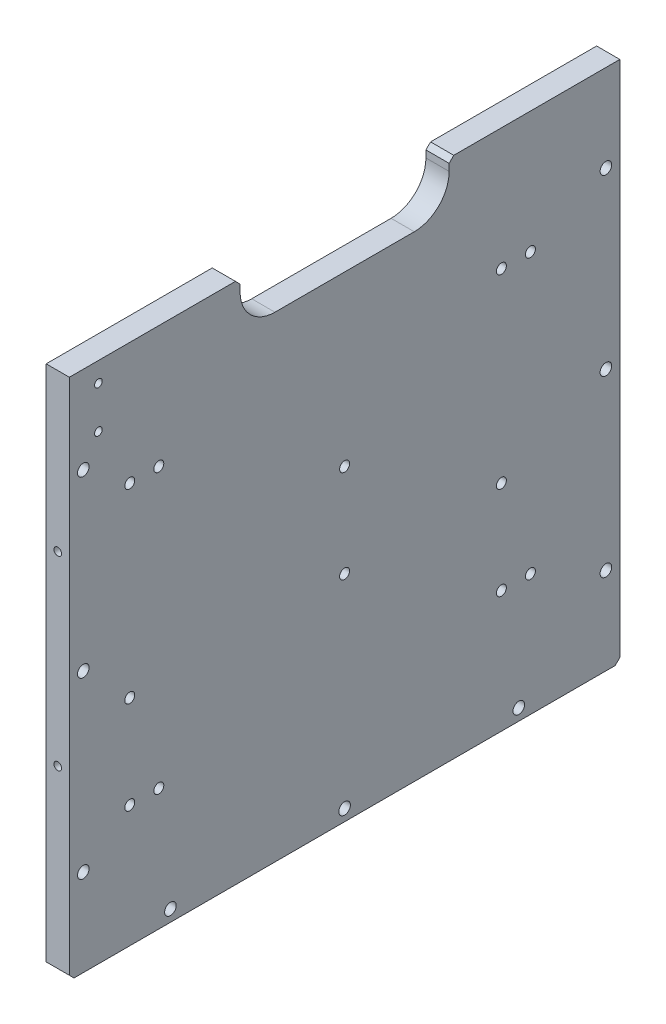
from build123d import *

# Parameters (mm, degrees)
SKETCH_1_W                  = 237
SKETCH_1_H                  = 250
EXTRUDE_1_DEPTH             = 5
MOVE_FACE_1_BY              = 17.5
MOVE_FACE_2_BY              = 7.5
HOLE_WIZARD_M4_1_AT_2_COUNT = 2
HOLE_WIZARD_M4_1_AT_2_PITCH = 80
HOLE_WIZARD_M4_2_D          = 3.3
HOLE_WIZARD_M6_1_D          = 5
HOLE_WIZARD_M6_2_D          = 5
CHAMFER_1_SIZE              = 2
CUT_EXTRUDE_1_DEPTH         = 71
CHAMFER_2_SIZE              = 2
HOLE_WIZARD_1_D             = 4.3
HOLE_WIZARD_1_CBORE_D       = 8
HOLE_WIZARD_1_CBORE_DEPTH   = 4.6
HOLE_WIZARD_1_2_D           = 4.3
HOLE_WIZARD_1_2_CBORE_D     = 8
HOLE_WIZARD_1_2_CBORE_DEPTH = 5


with BuildPart() as part:
    # 草图1 → 凸台-拉伸1 (new, symmetric)
    with BuildSketch(Plane(origin=(0, 0, 0), x_dir=(0, 0, -1), z_dir=(1, 0, 0))):
        Rectangle(SKETCH_1_W, SKETCH_1_H)
    extrude(amount=EXTRUDE_1_DEPTH, both=True)

    # Move Face 1: a face moved inward by 17.5
    extrude(part.faces().sort_by_distance((0, 125, 0))[0], amount=MOVE_FACE_1_BY, dir=(0, -1, 0), mode=Mode.SUBTRACT)

    # Move Face 2: a face moved inward by 7.5
    extrude(part.faces().sort_by_distance((0, -125, 0))[0], amount=MOVE_FACE_2_BY, dir=(0, 1, 0), mode=Mode.SUBTRACT)

    # 草图3 → M4 螺纹孔1 (revolve, cut)
    with BuildSketch(Plane(origin=(0, -40, 118.5), x_dir=(0, -1, 0), z_dir=(1, 0, 0))):
        Polygon((0, 0), (0, 11.091420021), (1.65, 10.1), (1.65, 0), align=None)
    hole_wizard_m4_1 = revolve(axis=Axis((0, -40, 124.85), (0, 0, -1)), mode=Mode.SUBTRACT)

    # M4 螺纹孔1 at 2: M4 螺纹孔1 ×2
    with Locations(*[(0, i * HOLE_WIZARD_M4_1_AT_2_PITCH, 0) for i in range(1, HOLE_WIZARD_M4_1_AT_2_COUNT)]):
        add(hole_wizard_m4_1, mode=Mode.SUBTRACT)

    # 镜向1: M4 螺纹孔1 across plane
    add(hole_wizard_m4_1.mirror(Plane.XY), mode=Mode.SUBTRACT)

    # 镜向1 copy 1 sketch → 镜向1 copy 1 (revolve, cut)
    with BuildSketch(Plane(origin=(0, 40, -118.5), x_dir=(0, -1, 0), z_dir=(1, 0, 0))):
        Polygon((0, 0), (0, -11.091420021), (1.65, -10.1), (1.65, 0), align=None)
    revolve(axis=Axis((0, 40, -124.85), (0, 0, -1)), mode=Mode.SUBTRACT)

    # M4 螺纹孔2 (through all)
    with Locations(Plane(origin=(5, 0, 0), x_dir=(0, 0, -1), z_dir=(1, 0, 0))):
        with Locations((-106, 99), (-106, 81)):
            Hole(HOLE_WIZARD_M4_2_D / 2)

    # M6 螺纹孔1 (through all)
    with Locations(Plane.ZY.offset(5)):
        with Locations((-112.5, 70), (-112.5, -5), (-112.5, -80)):
            hole_wizard_m6_1 = Hole(HOLE_WIZARD_M6_1_D / 2)

    # 镜向2: M6 螺纹孔1 across plane
    add(hole_wizard_m6_1.mirror(Plane.XY), mode=Mode.SUBTRACT)

    # M6 螺纹孔2 (through all)
    with Locations(Plane.ZY.offset(5)):
        with Locations((75, -112.5), (0, -112.5), (-75, -112.5)):
            Hole(HOLE_WIZARD_M6_2_D / 2)

    # 倒角1
    chamfer_1_edges = [part.edges().sort_by_distance(p)[0] for p in [
        (0, -117.5, -118.5),
        (0, -117.5, 118.5),
    ]]
    chamfer(chamfer_1_edges, length=CHAMFER_1_SIZE)

    # 草图11 → 切除-拉伸1 (cut)
    with BuildSketch(Plane.ZY.offset(5)):
        with BuildLine():
            Line((-45, 148.579976686), (45, 148.579976686))
            Line((45, 148.579976686), (45, 102.5))
            ThreePointArc((45, 102.5), (40.606601718, 91.893398282), (30, 87.5))
            Line((30, 87.5), (-30, 87.5))
            ThreePointArc((-30, 87.5), (-40.606601718, 91.893398282), (-45, 102.5))
            Line((-45, 102.5), (-45, 148.579976686))
        make_face()
    extrude(amount=-CUT_EXTRUDE_1_DEPTH, mode=Mode.SUBTRACT)

    # 倒角2
    chamfer_2_edges = [part.edges().sort_by_distance(p)[0] for p in [
        (0, 107.5, -45),
        (0, 107.5, 45),
    ]]
    chamfer(chamfer_2_edges, length=CHAMFER_2_SIZE)

    # Hole Wizard 1 (through all)
    with Locations(Plane.ZY.offset(5)):
        with Locations((-67.5, 55), (92.5, 55), (92.5, -65), (-67.5, -65), (-67.5, -25), (92.5, -25)):
            CounterBoreHole(HOLE_WIZARD_1_D / 2, HOLE_WIZARD_1_CBORE_D / 2, HOLE_WIZARD_1_CBORE_DEPTH)

    # Hole Wizard 1 2 (through all)
    with Locations(Plane.ZY.offset(5)):
        with Locations((80, 55), (-80, 55), (-80, -65), (80, -65), (0, -25), (0, 15)):
            CounterBoreHole(HOLE_WIZARD_1_2_D / 2, HOLE_WIZARD_1_2_CBORE_D / 2, HOLE_WIZARD_1_2_CBORE_DEPTH)


solid = part.part
